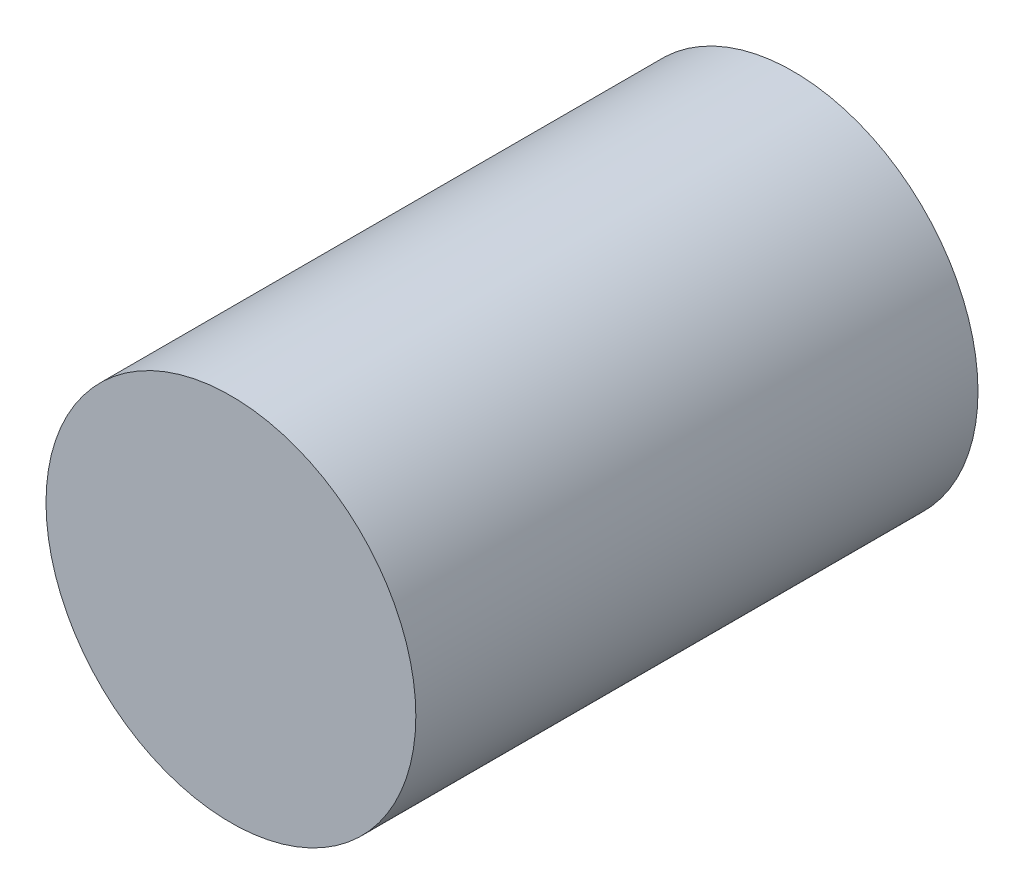
SolidWorks part; units mm, degrees
ref_plane "Front Plane" through (0, 0, 0) normal (0, 0, 1) x (1, 0, 0)
ref_plane "Top Plane" through (0, 0, 0) normal (0, 1, 0) x (1, 0, 0)
ref_plane "Right Plane" through (0, 0, 0) normal (1, 0, 0) x (0, 0, -1)
sketch "Sketch1" plane through (0, 0, 0) normal (0, 0, 1) x (1, 0, 0)
  circle A0 centre (432.9392, 69.2313) radius 12.5 construction
  circle A1 centre (432.9392, 69.2313) radius 12.5
extrude "Boss-Extrude1" add sketch "Sketch1" along normal blind 5 and the other way blind 33
